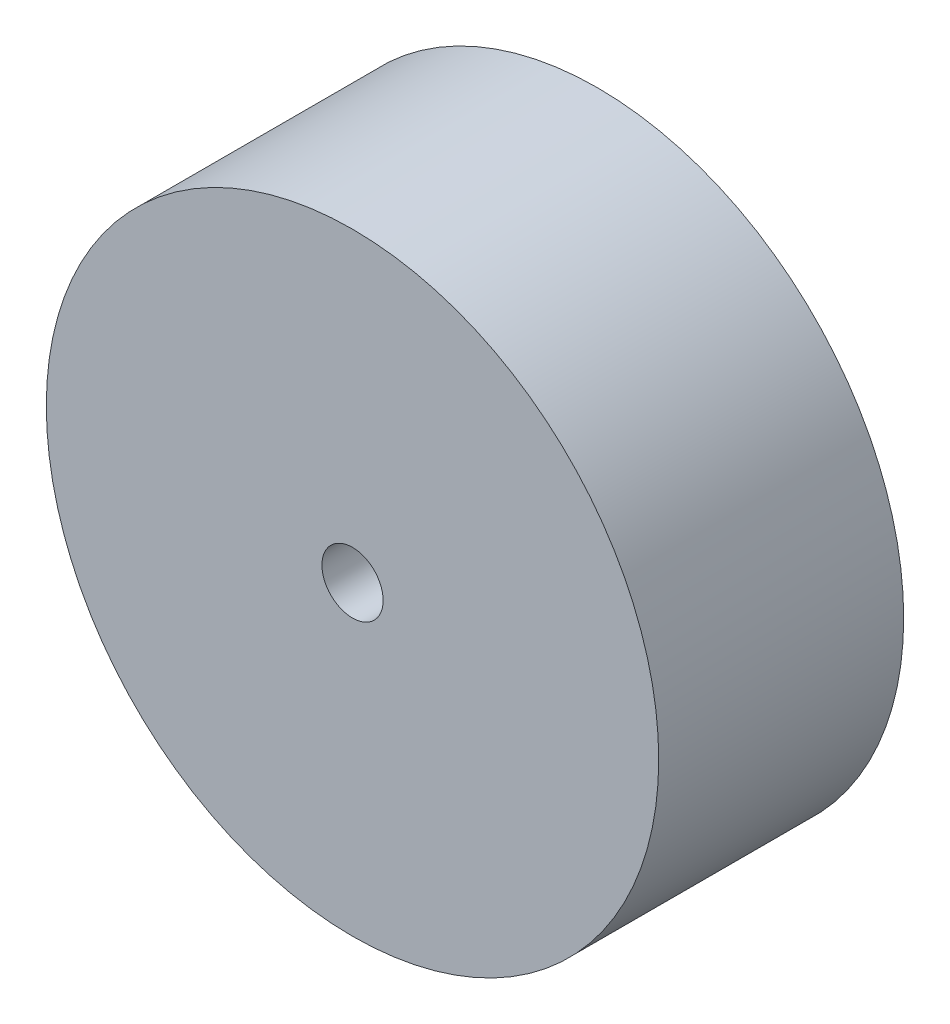
from build123d import *

# Parameters (mm, degrees)
SKETCH1_R           = 15
SKETCH1_R_2         = 1.5
BOSS_EXTRUDE1_DEPTH = 12


with BuildPart() as part:
    # Sketch1 → Boss-Extrude1 (new body)
    with BuildSketch(Plane.XY):
        Circle(SKETCH1_R)
        Circle(SKETCH1_R_2, mode=Mode.SUBTRACT)
    extrude(amount=BOSS_EXTRUDE1_DEPTH)


solid = part.part
